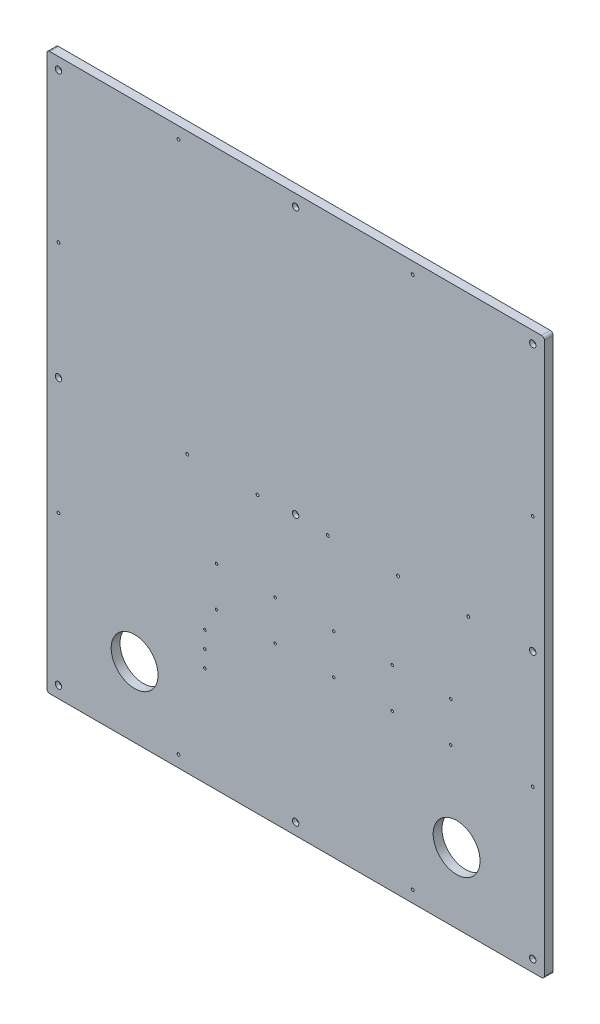
SolidWorks part; units mm, degrees
ref_plane "前视基准面" through (0, 0, 0) normal (0, 0, 1) x (1, 0, 0)
ref_plane "上视基准面" through (0, 0, 0) normal (0, 1, 0) x (1, 0, 0)
ref_plane "右视基准面" through (0, 0, 0) normal (1, 0, 0) x (0, 0, -1)
sketch "草图1" plane through (0, 0, 0) normal (0, 0, 1) x (1, 0, 0)
  line L1 (425, -475) -> (-425, -475)
  line L2 (425, -475) -> (425, 475)
  line L3 (425, 475) -> (-425, 475)
  line L4 (-425, -475) -> (-425, 475)
  line L5 (425, -475) -> (-425, 475) construction
  line L6 (425, 475) -> (-425, -475) construction
  point P0 (0, 0)
  dimension "D1" = 850
  dimension "D2" = 950
extrude "凸台-拉伸1" add sketch "草图1" along normal blind 15
fillet "圆角1" radius 5 4 edges at (-425, 475, 7.5) (425, 475, 7.5) (425, -475, 7.5) (-425, -475, 7.5)
hole_wizard "M5 螺纹孔1" positions "草图2" profile "草图3" tap size "M5" standard "GB" end condition up to next
sketch "草图2" plane through (0, 0, 15) normal (0, 0, 1) x (1, 0, 0)
  point P0 (265, -140.2)
  point P3 (265, -208.2)
sketch "草图3" plane through (265, -140.2, 15) normal (1, 0, 0) x (0, -1, 0)
  line L0 (0, 0) -> (0, 15)
  line L1 (0, 15) -> (2.1, 15)
  line L2 (2.1, 15) -> (2.1, 0)
  line L5 (2.1, 0) -> (0, 0)
  line L11 (0, -6.35) -> (0, 107.95) construction
  dimension "通孔螺纹孔钻头直径" = 4.2
  dimension "通孔螺纹孔钻头深度" = 15
cosmetic thread "孔螺蚊线1" parameters "D2"=5
cosmetic thread "孔螺蚊线2" parameters "D2"=5
pattern_linear "阵列(线性)1" count 5 spacing 100 along (-1, 0, 0) of "M5 螺纹孔1"
hole_wizard "M6 螺纹孔1" positions "草图4" profile "草图5" tap size "M6" standard "GB" end condition up to next
sketch "草图4" plane through (0, 0, 15) normal (0, 0, 1) x (1, 0, 0)
  point P0 (-185, -3.4)
  point P3 (-65, -3.4)
  point P6 (55, -3.4)
  point P9 (175, -3.4)
  point P12 (295, -3.4)
sketch "草图5" plane through (-185, -3.4, 15) normal (1, 0, 0) x (0, -1, 0)
  line L0 (0, 0) -> (0, 15)
  line L1 (0, 15) -> (2.5, 15)
  line L2 (2.5, 15) -> (2.5, 0)
  line L5 (2.5, 0) -> (0, 0)
  line L11 (0, -6.35) -> (0, 107.95) construction
  dimension "通孔螺纹孔钻头直径" = 5
  dimension "通孔螺纹孔钻头深度" = 15
cosmetic thread "孔螺蚊线4" parameters "D2"=6
cosmetic thread "孔螺蚊线5" parameters "D2"=6
cosmetic thread "孔螺蚊线6" parameters "D2"=6
cosmetic thread "孔螺蚊线7" parameters "D2"=6
cosmetic thread "孔螺蚊线8" parameters "D2"=6
sketch "草图6" plane through (0, 0, 15) normal (0, 0, 1) x (1, 0, 0)
  line L0 (-420, -475) -> (420, -475) construction
  line L1 (-425, 470) -> (-425, -470) construction
  line L2 (0, -475) -> (0, -373.8857) construction
  circle A0 centre (-275, -355) radius 40
  circle A1 centre (275, -355) radius 40
  dimension "D1" = 80
  dimension "D2" = 120
  dimension "D3" = 150
extrude "切除-拉伸1" cut sketch "草图6" against normal up to next
hole_wizard "M5 螺纹孔2" positions "草图7" profile "草图8" tap size "M5" standard "GB" end condition up to next
sketch "草图7" plane through (0, 0, 15) normal (0, 0, 1) x (1, 0, 0)
  line L0 (-155, -248) -> (-155, -276.5) construction
  line L1 (-155, -276.5) -> (-155, -305) construction
  line L6 (-425, 470) -> (-425, -470) construction
  line L7 (-420, -475) -> (420, -475) construction
  point P0 (-155, -248)
  point P2 (-155, -276.5)
  point P4 (-155, -305)
  dimension "D1" = 28.5
  dimension "D2" = 270
  dimension "D3" = 170
sketch "草图8" plane through (-155, -248, 15) normal (1, 0, 0) x (0, -1, 0)
  line L0 (0, 0) -> (0, 15)
  line L1 (0, 15) -> (2.1, 15)
  line L2 (2.1, 15) -> (2.1, 0)
  line L5 (2.1, 0) -> (0, 0)
  line L11 (0, -6.35) -> (0, 107.95) construction
  dimension "通孔螺纹孔钻头直径" = 4.2
  dimension "通孔螺纹孔钻头深度" = 15
cosmetic thread "孔螺蚊线9" parameters "D2"=5
cosmetic thread "孔螺蚊线10" parameters "D2"=5
cosmetic thread "孔螺蚊线11" parameters "D2"=5
hole_wizard "打孔尺寸(%根据)内六角圆柱头螺钉的类型1" positions "草图9" profile "草图10" counterbore size "M6" standard "GB" end condition up to next
sketch "草图9" plane through (0, 0, 15) normal (0, 0, 1) x (1, 0, 0)
  point P0 (-405, -455)
  point P3 (0, -455)
  point P6 (405, -455)
  point P9 (0, 0)
  point P12 (-405, 0)
  point P15 (-405, 455)
  point P18 (0, 455)
  point P21 (405, 455)
  point P24 (405, 0)
sketch "草图10" plane through (-405, -455, 15) normal (1, 0, 0) x (0, -1, 0)
  line L0 (0, 0) -> (0, 15)
  line L1 (0, 15) -> (3.3, 15)
  line L3 (3.3, 15) -> (3.3, 6.8)
  line L4 (3.3, 6.8) -> (5.5, 6.8)
  line L5 (5.5, 6.8) -> (5.5, 0)
  line L7 (5.5, 0) -> (0, 0)
  line L11 (0, -6.35) -> (0, 107.95) construction
  dimension "通孔孔直径" = 6.6
  dimension "通孔孔深度" = 15
  dimension "柱形沉头孔直径" = 11
  dimension "柱形沉头孔深度" = 6.8
hole_wizard "M6 螺纹孔2" positions "草图11" profile "草图12" tap size "M6" standard "GB" end condition up to next
sketch "草图11" plane through (0, 0, 15) normal (0, 0, 1) x (1, 0, 0)
  point P0 (-405, 200)
  point P3 (-405, -200)
  point P6 (-200, -455)
  point P9 (200, -455)
  point P12 (405, -200)
  point P15 (405, 200)
  point P18 (200, 455)
  point P21 (-200, 455)
sketch "草图12" plane through (-405, 200, 15) normal (1, 0, 0) x (0, -1, 0)
  line L0 (0, 0) -> (0, 15)
  line L1 (0, 15) -> (2.5, 15)
  line L2 (2.5, 15) -> (2.5, 0)
  line L5 (2.5, 0) -> (0, 0)
  line L11 (0, -6.35) -> (0, 107.95) construction
  dimension "通孔螺纹孔钻头直径" = 5
  dimension "通孔螺纹孔钻头深度" = 15
cosmetic thread "孔螺蚊线12" parameters "D2"=6
cosmetic thread "孔螺蚊线13" parameters "D2"=6
cosmetic thread "孔螺蚊线14" parameters "D2"=6
cosmetic thread "孔螺蚊线15" parameters "D2"=6
cosmetic thread "孔螺蚊线16" parameters "D2"=6
cosmetic thread "孔螺蚊线17" parameters "D2"=6
cosmetic thread "孔螺蚊线18" parameters "D2"=6
cosmetic thread "孔螺蚊线19" parameters "D2"=6
